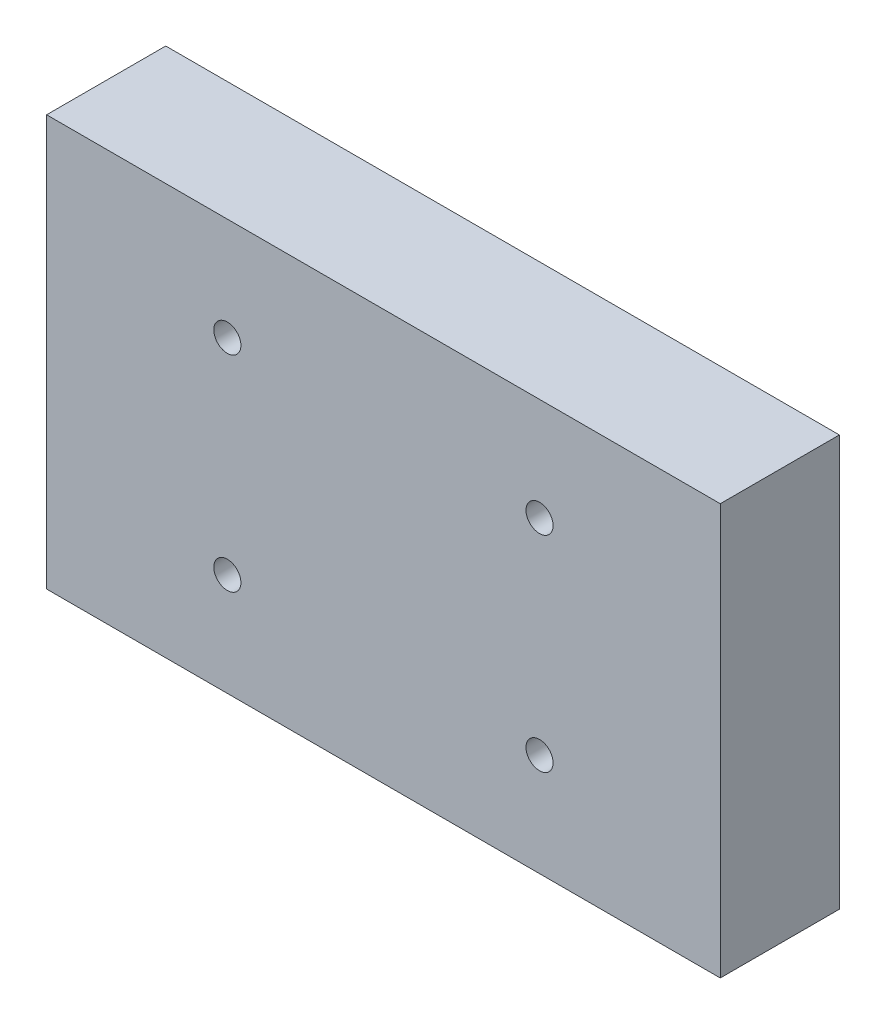
SolidWorks part; units mm, degrees
ref_plane "Front Plane" through (0, 0, 0) normal (0, 0, 1) x (1, 0, 0)
ref_plane "Top Plane" through (0, 0, 0) normal (0, 1, 0) x (1, 0, 0)
ref_plane "Right Plane" through (0, 0, 0) normal (1, 0, 0) x (0, 0, -1)
other "Configuration Table"
sketch "Sketch1" plane through (0, 0, 0) normal (0, 0, 1) x (1, 0, 0)
  line L1 (41, 25) -> (-41, 25)
  line L2 (41, 25) -> (41, -25)
  line L3 (41, -25) -> (-41, -25)
  line L4 (-41, 25) -> (-41, -25)
  line L5 (41, 25) -> (-41, -25) construction
  line L6 (41, -25) -> (-41, 25) construction
  line L7 (19, 12.5) -> (-19, 12.5) construction
  line L8 (19, 12.5) -> (19, -12.5) construction
  line L9 (19, -12.5) -> (-19, -12.5) construction
  line L10 (-19, 12.5) -> (-19, -12.5) construction
  line L11 (19, 12.5) -> (-19, -12.5) construction
  line L12 (19, -12.5) -> (-19, 12.5) construction
  point P0 (0, 0)
  point P6 (0, 0)
  dimension "D1" = 50
  dimension "D2" = 82
  dimension "D3" = 38
  dimension "D4" = 25
extrude "Boss-Extrude1" add sketch "Sketch1" along normal blind 16
sketch "Sketch3" plane through (0, 0, 0) normal (0, 0, -1) x (-1, 0, 0)
  line L0 (-19, -12.5) -> (19, -12.5) construction
  line L1 (-19, 12.5) -> (-19, -12.5) construction
  line L2 (-19, 12.5) -> (19, 12.5) construction
  line L3 (19, 12.5) -> (19, -12.5) construction
  line L4 (-19, -12.5) -> (19, -12.5) construction
  line L5 (-19, 12.5) -> (-19, -12.5) construction
  line L6 (-19, 12.5) -> (19, 12.5) construction
  line L7 (19, 12.5) -> (19, -12.5) construction
hole_wizard "M4 Tapped Hole1" positions "3DSketch7" profile "Sketch8" tap size "M4" standard "GB" end condition through all
sketch3d "3DSketch7"
  point P4 (19, 12.5, 0)
sketch "Sketch8" plane through (19, 12.5, 0) normal (1, 0, 0) x (0, 1, 0)
  line L0 (0, 0) -> (0, 16)
  line L1 (0, 16) -> (1.65, 16)
  line L2 (1.65, 16) -> (1.65, 0)
  line L5 (1.65, 0) -> (0, 0)
  line L11 (0, -6.35) -> (0, 107.95) construction
  dimension "通孔螺纹孔钻头直径" = 3.3
  dimension "通孔螺纹孔钻头深度" = 16
cosmetic thread "Cosmetic thread 1" parameters "D2"=4
pattern_linear "LPattern1" count 2 spacing 38 along (-1, 0, 0) count 2 spacing 25 along (0, -1, 0) of "M4 Tapped Hole1"
chamfer "Chamfer1" distance 1.5 angle 45 4 edges at (-41, 0, 0) (0, -25, 0) (0, 25, 0) (41, 0, 0)
